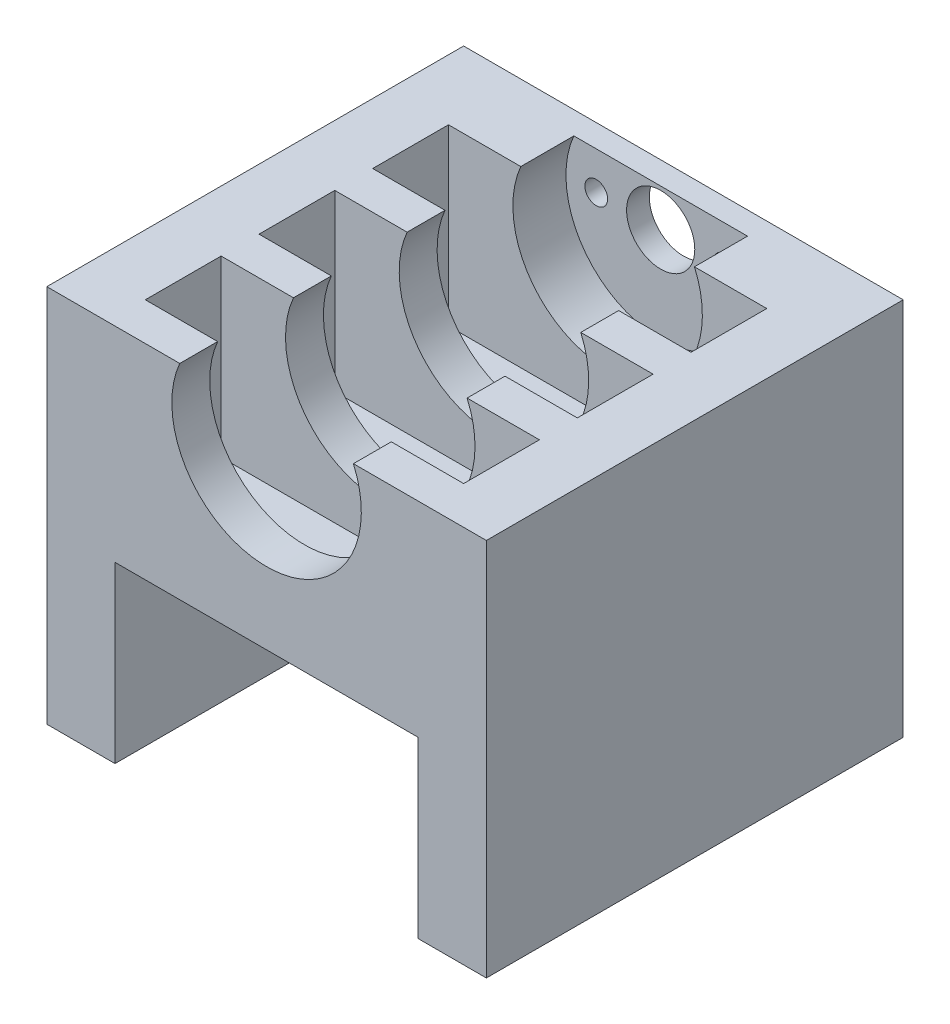
SolidWorks part; units mm, degrees
ref_plane "Front Plane" through (0, 0, 0) normal (0, 0, 1) x (1, 0, 0)
ref_plane "Top Plane" through (0, 0, 0) normal (0, 1, 0) x (1, 0, 0)
ref_plane "Right Plane" through (0, 0, 0) normal (1, 0, 0) x (0, 0, -1)
sketch "Sketch1" plane through (0, 0, 0) normal (0, 0, 1) x (1, 0, 0)
  line L1 (-29, 25) -> (29, 25)
  line L2 (-29, 25) -> (-29, -25)
  line L3 (-29, -25) -> (29, -25)
  line L4 (29, 25) -> (29, -25)
  line L5 (-29, 25) -> (29, -25) construction
  line L6 (-29, -25) -> (29, 25) construction
  point P0 (0, 0)
  dimension "D1" = 58
  dimension "D2" = 50
extrude "Boss-Extrude1" add sketch "Sketch1" along normal blind 55
sketch "Sketch3" plane through (0, 0, 0) normal (0, 0, -1) x (-1, 0, 0)
  line L0 (29, -25) -> (-29, -25) construction
  circle A0 centre (0, 20) radius 4.5
  circle A1 centre (-8.5, 20) radius 1.5
  circle A2 centre (8.5, 20) radius 1.5
  dimension "D1" = 45
  dimension "D2" = 8.5
  dimension "D3" = 8.5
extrude "Cut-Extrude2" cut sketch "Sketch3" against normal blind 5
sketch "Sketch2" plane through (0, 0, 55) normal (0, 0, 1) x (1, 0, 0)
  line L0 (-29, -25) -> (29, -25) construction
  circle A0 centre (0, 20) radius 12.5
  dimension "D1" = 45
extrude "Cut-Extrude1" cut sketch "Sketch2" against normal blind 52
sketch "Sketch4" plane through (0, 0, 0) normal (0, 0, -1) x (-1, 0, 0)
  line L0 (29, -25) -> (-29, -25) construction
  line L1 (-20, -48) -> (20, -48)
  line L2 (-20, -48) -> (-20, -2)
  line L3 (-20, -2) -> (20, -2)
  line L4 (20, -48) -> (20, -2)
  line L5 (-20, -48) -> (20, -2) construction
  line L6 (-20, -2) -> (20, -48) construction
  point P0 (0, -25)
  dimension "D1" = 23
  dimension "D2" = 40
extrude "Cut-Extrude3" cut sketch "Sketch4" against normal blind 70
sketch "Sketch5" plane through (0, -25, 0) normal (0, -1, 0) x (1, 0, 0)
  line L0 (24.5, 47) -> (24.5, 8) construction
  line L1 (20, 55) -> (29, 55) construction
  line L2 (20, 0) -> (29, 0) construction
  line L3 (-24.5, 47) -> (-24.5, 8) construction
  line L4 (-29, 55) -> (-20, 55) construction
  line L5 (-29, 0) -> (-20, 0) construction
  dimension "D1" = 8
  dimension "D2" = 8
  dimension "D3" = 8
  dimension "D4" = 8
hole_wizard "M4 Tapped Hole1" positions "Sketch6" profile "Sketch7" tap size "M4" standard "GB"
sketch "Sketch6" plane through (0, -25, 0) normal (0, -1, 0) x (-1, 0, 0)
  line L0 (-24.5, -47) -> (-24.5, -8) construction
  point P0 (24.5, -47)
  point P3 (24.5, -8)
  point P6 (-24.5, -8)
  point P9 (-24.5, -47)
sketch "Sketch7" plane through (-24.5, -25, 47) normal (1, 0, 0) x (0, 0, -1)
  line L0 (0, 0) -> (0, 11.0914)
  line L1 (0, 11.0914) -> (1.65, 10.1)
  line L2 (1.65, 10.1) -> (1.65, 0)
  line L5 (1.65, 0) -> (0, 0)
  line L10 (0, 11.0914) -> (-1.65, 10.1) construction
  line L11 (0, -6.35) -> (0, 107.95) construction
  dimension "螺纹孔钻头直径" = 3.3
  dimension "螺纹孔钻头深度" = 10.1
  dimension "导头角度" = 118
cosmetic thread "CosmeticThread1" parameters "D1"=8, "D2"=4
cosmetic thread "CosmeticThread2" parameters "D1"=8, "D2"=4
cosmetic thread "CosmeticThread3" parameters "D1"=8, "D2"=4
cosmetic thread "CosmeticThread4" parameters "D1"=8, "D2"=4
sketch "Sketch8" plane through (0, 25, 0) normal (0, 1, 0) x (1, 0, 0)
  line L0 (29, -55) -> (29, 0) construction
  line L1 (-21, -20) -> (21, -20)
  line L2 (-21, -20) -> (-21, -10)
  line L3 (-21, -10) -> (21, -10)
  line L4 (21, -20) -> (21, -10)
  line L5 (-21, -20) -> (21, -10) construction
  line L6 (-21, -10) -> (21, -20) construction
  line L7 (-29, -55) -> (-29, 0) construction
  line L8 (29, 0) -> (-29, 0) construction
  line L9 (-21, -35) -> (21, -35)
  line L10 (-21, -35) -> (-21, -25)
  line L11 (-21, -25) -> (21, -25)
  line L12 (21, -35) -> (21, -25)
  line L13 (-21, -35) -> (21, -25) construction
  line L14 (-21, -25) -> (21, -35) construction
  line L15 (-21, -50) -> (21, -50)
  line L16 (-21, -50) -> (-21, -40)
  line L17 (-21, -40) -> (21, -40)
  line L18 (21, -50) -> (21, -40)
  line L19 (-21, -50) -> (21, -40) construction
  line L20 (-21, -40) -> (21, -50) construction
  line L21 (0, -15) -> (0, -30) construction
  point P0 (0, -15)
  point P13 (0, -30)
  point P18 (0, -45)
  dimension "D1" = 8
  dimension "D2" = 8
  dimension "D3" = 10
  dimension "D4" = 10
  dimension "D6" = 15
  dimension "D5" = 3
extrude "Cut-Extrude4" cut sketch "Sketch8" against normal blind 23
